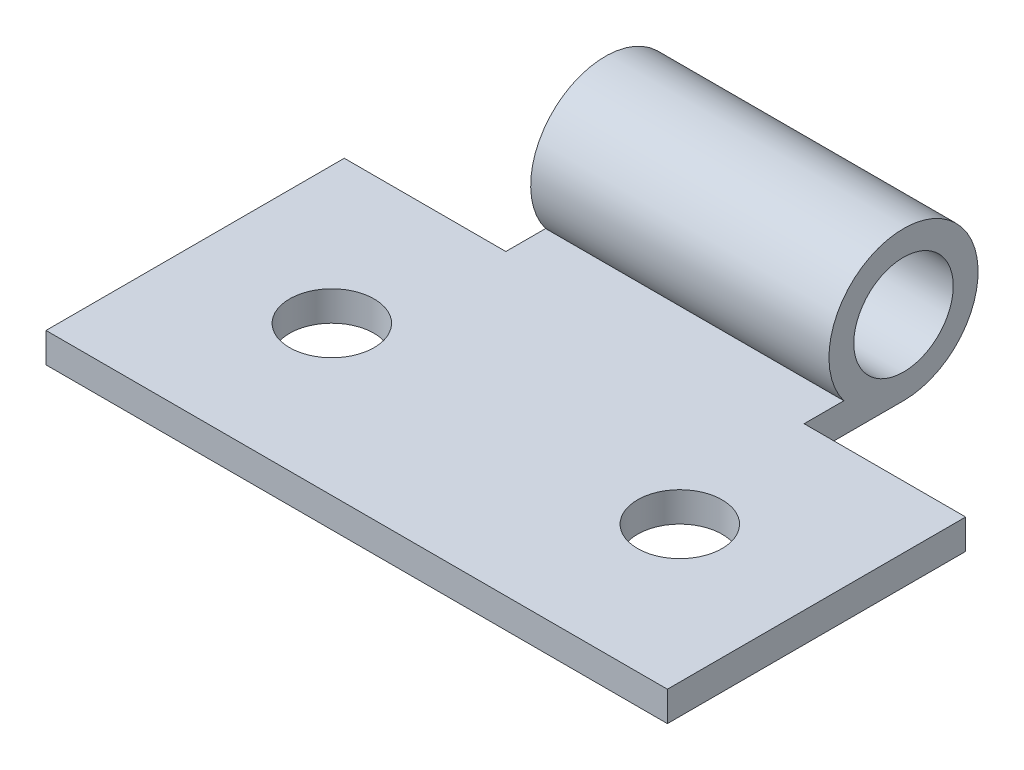
from build123d import *

# Parameters (mm, degrees)
SKETCH_1_R          = 2
EXTRUDE_1_DEPTH     = 12.5
SKETCH_2_R          = 1.7
CUT_EXTRUDE_1_DEPTH = 21.863604674
CUT_EXTRUDE_2_DEPTH = 6.5


with BuildPart() as part:
    # 草图1 → 凸台-拉伸1 (new, symmetric)
    with BuildSketch(Plane(origin=(0, 0, 0), x_dir=(0, 0, -1), z_dir=(1, 0, 0))):
        with BuildLine():
            Line((0, -3), (-16, -3))
            Line((-16, -3), (-16, -1.8))
            Line((-16, -1.8), (-2.4, -1.8))
            ThreePointArc((-2.4, -1.8), (1.341640786, 2.683281573), (0, -3))
        make_face()
        Circle(SKETCH_1_R, mode=Mode.SUBTRACT)
    extrude(amount=EXTRUDE_1_DEPTH, both=True)

    # 草图2 → 切除-拉伸1 (cut, through all)
    with BuildSketch(Plane(origin=(0, -1.8, 0), x_dir=(1, 0, 0), z_dir=(0, 1, 0))):
        with Locations(Location((-7, -10, 0), (0, 0, 270))):
            Circle(SKETCH_2_R)
        with Locations(Location((7, -10, 0), (0, 0, 270))):
            Circle(SKETCH_2_R)
    extrude(amount=-CUT_EXTRUDE_1_DEPTH, mode=Mode.SUBTRACT)

    # 草图3 → 切除-拉伸2 (cut)
    with BuildSketch(Plane(origin=(12.5, 0, 0), x_dir=(0, 0, -1), z_dir=(1, 0, 0))):
        with BuildLine():
            Line((-4, -3), (0, -3))
            ThreePointArc((0, -3), (1.341640786, 2.683281573), (-2.4, -1.8))
            Line((-2.4, -1.8), (-4, -1.8))
            Line((-4, -1.8), (-4, -3))
        make_face()
    cut_extrude_2 = extrude(amount=-CUT_EXTRUDE_2_DEPTH, mode=Mode.SUBTRACT)

    # 镜向1: 切除-拉伸2 across plane
    add(cut_extrude_2.mirror(Plane(origin=(0, 0, 0), x_dir=(0, 0, 1), z_dir=(1, 0, 0))), mode=Mode.SUBTRACT)


solid = part.part
